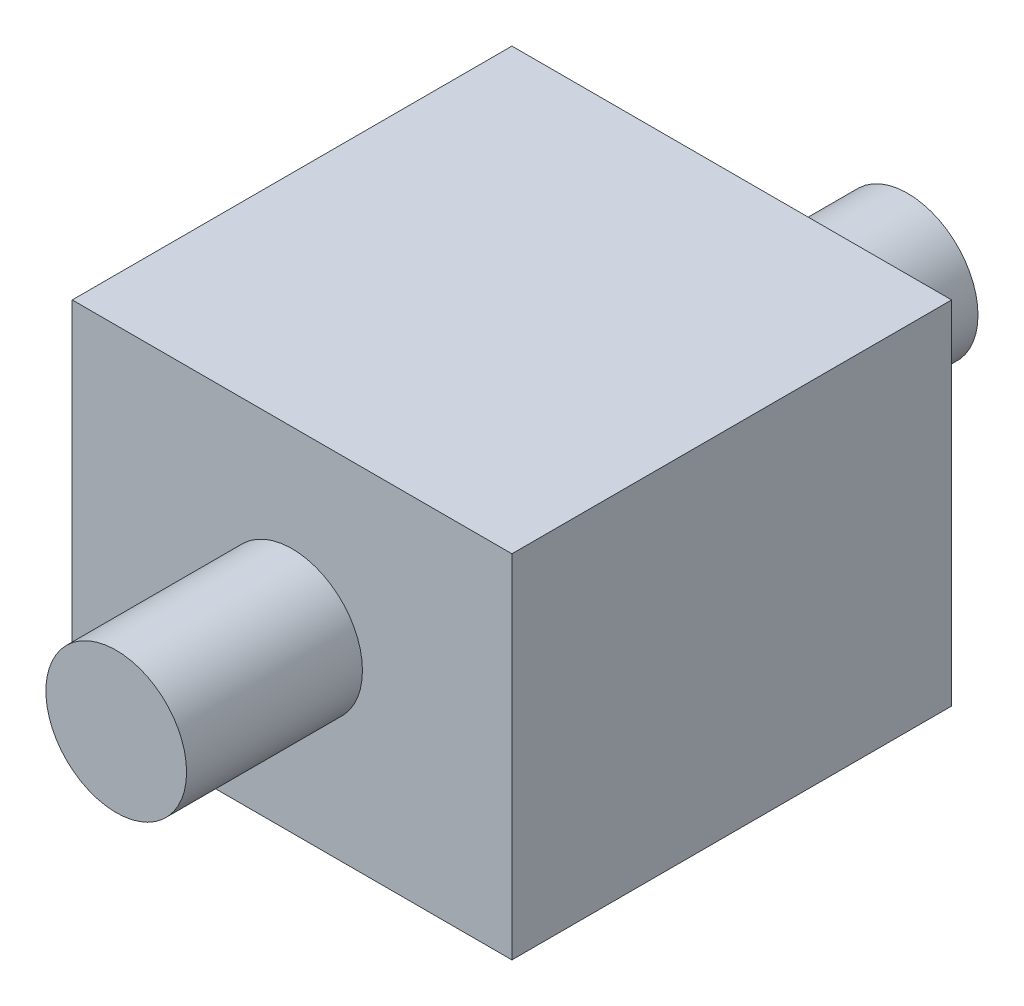
SolidWorks part; units mm, degrees
material "AISI 1045 Steel, cold drawn"
ref_plane "Front Plane" through (0, 0, 0) normal (0, 0, 1) x (1, 0, 0)
ref_plane "Top Plane" through (0, 0, 0) normal (0, 1, 0) x (1, 0, 0)
ref_plane "Right Plane" through (0, 0, 0) normal (1, 0, 0) x (0, 0, -1)
sketch "Sketch1" plane through (0, 0, 0) normal (0, 1, 0) x (1, 0, 0)
  line L1 (-12.5, -12.5) -> (12.5, -12.5)
  line L2 (-12.5, -12.5) -> (-12.5, 12.5)
  line L3 (-12.5, 12.5) -> (12.5, 12.5)
  line L4 (12.5, -12.5) -> (12.5, 12.5)
  line L5 (-12.5, -12.5) -> (12.5, 12.5) construction
  line L6 (-12.5, 12.5) -> (12.5, -12.5) construction
  point P0 (0, 0)
  dimension "D1" = 25
  dimension "D2" = 25
extrude "Boss-Extrude1" add sketch "Sketch1" along normal blind 20
sketch "Sketch2" plane through (0, 0, 12.5) normal (0, 0, 1) x (1, 0, 0)
  line L0 (12.5, 20) -> (-12.5, 0) construction
  line L1 (13.75, 0) -> (-13.75, 0) construction
  circle A0 centre (0, 10) radius 4
  dimension "D1" = 8
extrude "Boss-Extrude2" add sketch "Sketch2" along normal blind 10
mirror "Mirror1" about plane through (0, 0, 0) normal (0, 0, 1) of "Boss-Extrude2"
